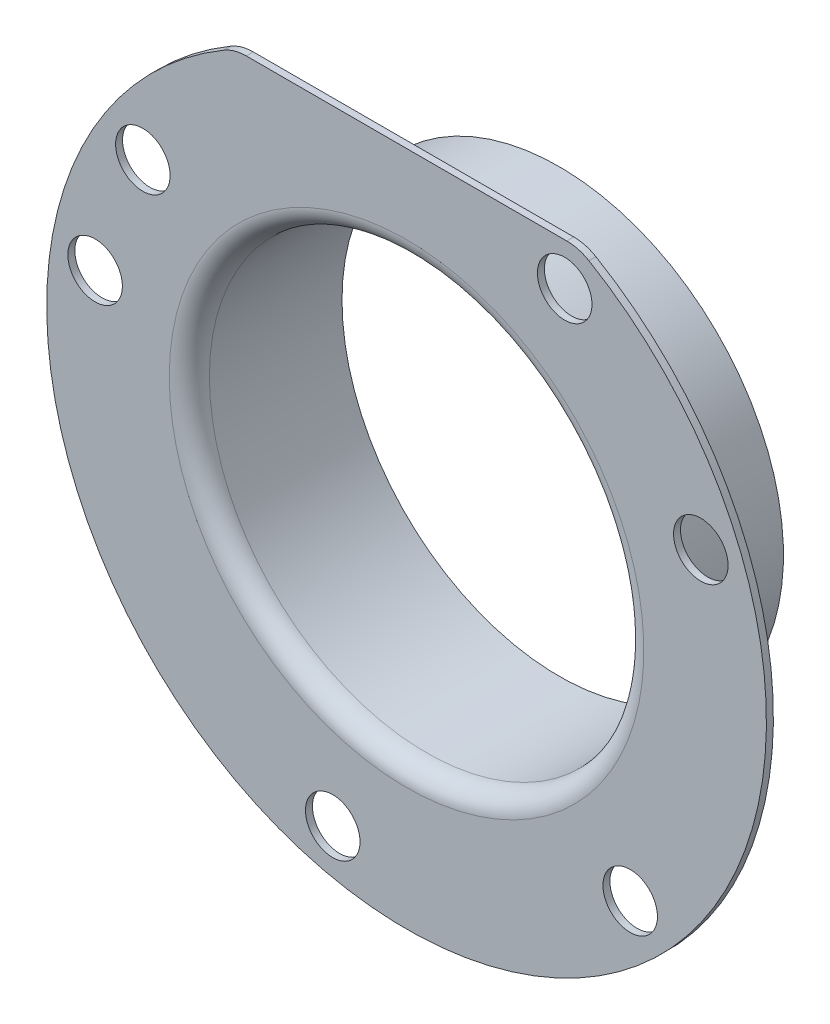
from build123d import *

# Parameters (mm, degrees)
CUT_EXTRUDE1_REACH = 123.809
SKETCH2_R          = 6.25
SKETCH2_W          = 90
SKETCH2_H          = 12
FILLET1_R          = 10


with BuildPart() as part:
    # Sketch1 → Revolve-Thin2 (revolve)
    with BuildSketch(Plane(origin=(0, 0, 0), x_dir=(0, 0, -1), z_dir=(1, 0, 0)), mode=Mode.PRIVATE) as revolve_thin2_sk:
        with BuildLine():
            Line((0, 49.8), (-30.4, 49.8))
            ThreePointArc((-30.4, 49.8), (-33.652691193, 51.147308807), (-35, 54.4))
            Line((-35, 54.4), (-35, 82.5))
            Line((-35, 82.5), (-33.4, 82.5))
            Line((-33.4, 82.5), (-33.4, 54.4))
            ThreePointArc((-33.4, 54.4), (-32.521320344, 52.278679656), (-30.4, 51.4))
            Line((-30.4, 51.4), (0, 51.4))
            Line((0, 51.4), (0, 49.8))
        make_face()
    revolve(revolve_thin2_sk.sketch.rotate(Axis((0, 0, 0), (0, 0, 1)), 90), axis=Axis((0, 0, 0), (0, 0, 1)))

    # Sketch2 → Cut-Extrude1 (cut, up to next)
    with BuildSketch(Plane.XY.offset(35), mode=Mode.PRIVATE) as cut_extrude1_sk1:
        with Locations((-60.4567221, 40.015431435)):
            Circle(SKETCH2_R)
    cut_extrude1_tool1 = extrude(cut_extrude1_sk1.sketch, amount=-CUT_EXTRUDE1_REACH, mode=Mode.PRIVATE) & part.part
    # Sketch2 → Cut-Extrude1 (cut, up to next)
    with BuildSketch(Plane.XY.offset(35), mode=Mode.PRIVATE) as cut_extrude1_sk2:
        with Locations((36.25, 62.786841774)):
            Circle(SKETCH2_R)
    cut_extrude1_tool2 = extrude(cut_extrude1_sk2.sketch, amount=-CUT_EXTRUDE1_REACH, mode=Mode.PRIVATE) & part.part
    # Sketch2 → Cut-Extrude1 (cut, up to next)
    with BuildSketch(Plane.XY.offset(35), mode=Mode.PRIVATE) as cut_extrude1_sk3:
        with Locations((67.455273679, 26.571338938)):
            Circle(SKETCH2_R)
    cut_extrude1_tool3 = extrude(cut_extrude1_sk3.sketch, amount=-CUT_EXTRUDE1_REACH, mode=Mode.PRIVATE) & part.part
    # Sketch2 → Cut-Extrude1 (cut, up to next)
    with BuildSketch(Plane.XY.offset(35), mode=Mode.PRIVATE) as cut_extrude1_sk4:
        with Locations((51.265241636, -51.265241636)):
            Circle(SKETCH2_R)
    cut_extrude1_tool4 = extrude(cut_extrude1_sk4.sketch, amount=-CUT_EXTRUDE1_REACH, mode=Mode.PRIVATE) & part.part
    # Sketch2 → Cut-Extrude1 (cut, up to next)
    with BuildSketch(Plane.XY.offset(35), mode=Mode.PRIVATE) as cut_extrude1_sk5:
        with Locations((-16.92478888, -70.496819229)):
            Circle(SKETCH2_R)
    cut_extrude1_tool5 = extrude(cut_extrude1_sk5.sketch, amount=-CUT_EXTRUDE1_REACH, mode=Mode.PRIVATE) & part.part
    # Sketch2 → Cut-Extrude1 (cut, up to next)
    with BuildSketch(Plane.XY.offset(35), mode=Mode.PRIVATE) as cut_extrude1_sk6:
        with Locations((-71.398562093, 12.589492881)):
            Circle(SKETCH2_R)
    cut_extrude1_tool6 = extrude(cut_extrude1_sk6.sketch, amount=-CUT_EXTRUDE1_REACH, mode=Mode.PRIVATE) & part.part
    # Sketch2 → Cut-Extrude1 (cut, up to next)
    with BuildSketch(Plane.XY.offset(35), mode=Mode.PRIVATE) as cut_extrude1_sk7:
        with Locations((0, 78.5)):
            Rectangle(SKETCH2_W, SKETCH2_H)
    cut_extrude1_tool7 = extrude(cut_extrude1_sk7.sketch, amount=-CUT_EXTRUDE1_REACH, mode=Mode.PRIVATE) & part.part
    add(cut_extrude1_tool1.solids().sort_by_distance((-60.456722, 40.015431, 35))[0], mode=Mode.SUBTRACT)
    add(cut_extrude1_tool2.solids().sort_by_distance((36.25, 62.786842, 35))[0], mode=Mode.SUBTRACT)
    add(cut_extrude1_tool3.solids().sort_by_distance((67.455274, 26.571339, 35))[0], mode=Mode.SUBTRACT)
    add(cut_extrude1_tool4.solids().sort_by_distance((51.265242, -51.265242, 35))[0], mode=Mode.SUBTRACT)
    add(cut_extrude1_tool5.solids().sort_by_distance((-16.924789, -70.496819, 35))[0], mode=Mode.SUBTRACT)
    add(cut_extrude1_tool6.solids().sort_by_distance((-71.398562, 12.589493, 35))[0], mode=Mode.SUBTRACT)
    add(cut_extrude1_tool7.solids().sort_by_distance((0, 78.5, 35))[0], mode=Mode.SUBTRACT)

    # Fillet1
    fillet1_edges = [part.edges().sort_by_distance(p)[0] for p in [
        (-39.37003937, 72.5, 34.2),
        (39.37003937, 72.5, 34.2),
    ]]
    fillet(fillet1_edges, radius=FILLET1_R)


solid = part.part
